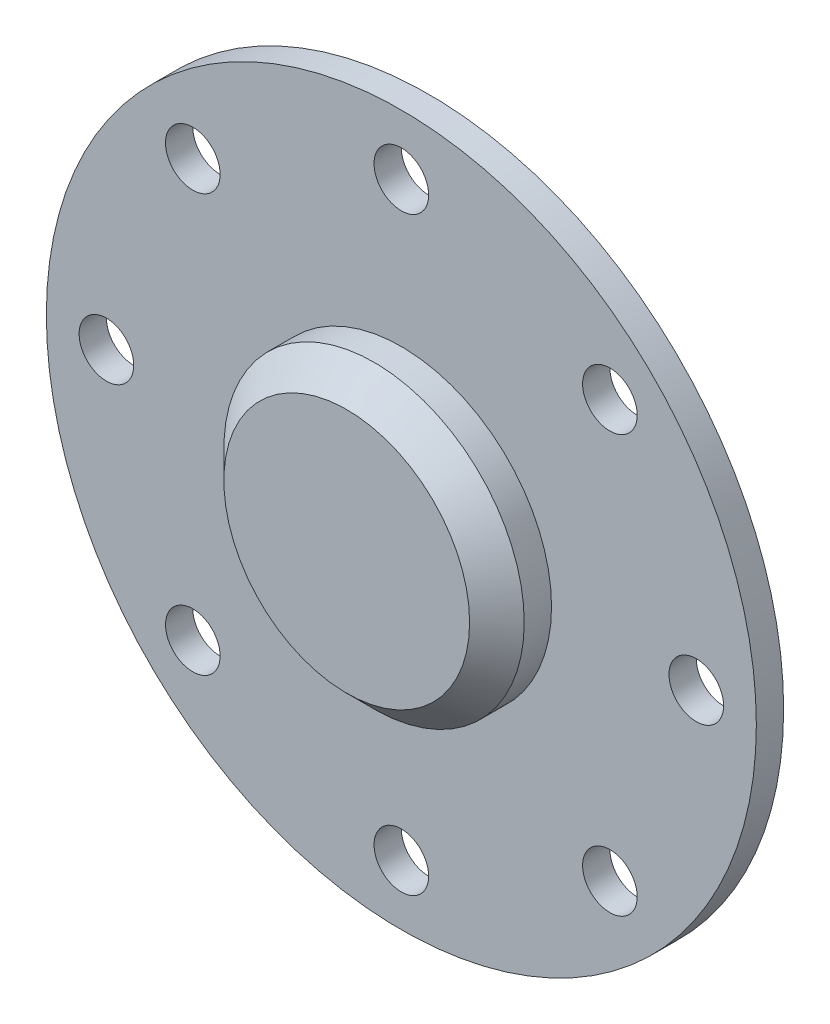
from build123d import *

# Parameters (mm, degrees)
SKETCH_1_R          = 130
SKETCH_1_R_2        = 10
EXTRUDE_1_DEPTH     = 10
SKETCH_2_R          = 55
EXTRUDE_2_DEPTH     = 20
SKETCH_3_R          = 45
CUT_EXTRUDE_1_DEPTH = 20
CHAMFER_1_SIZE      = 10


with BuildPart() as part:
    # 草图1 → 凸台-拉伸1 (new body)
    with BuildSketch(Plane.XY):
        Circle(SKETCH_1_R)
        with Locations((0, 108)):
            Circle(SKETCH_1_R_2, mode=Mode.SUBTRACT)
        with Locations((76.367532368, 76.367532368)):
            Circle(SKETCH_1_R_2, mode=Mode.SUBTRACT)
        with Locations((108, 0)):
            Circle(SKETCH_1_R_2, mode=Mode.SUBTRACT)
        with Locations((76.367532368, -76.367532368)):
            Circle(SKETCH_1_R_2, mode=Mode.SUBTRACT)
        with Locations((0, -108)):
            Circle(SKETCH_1_R_2, mode=Mode.SUBTRACT)
        with Locations((-76.367532368, -76.367532368)):
            Circle(SKETCH_1_R_2, mode=Mode.SUBTRACT)
        with Locations((-108, 0)):
            Circle(SKETCH_1_R_2, mode=Mode.SUBTRACT)
        with Locations((-76.367532368, 76.367532368)):
            Circle(SKETCH_1_R_2, mode=Mode.SUBTRACT)
    extrude(amount=EXTRUDE_1_DEPTH)

    # 草图2 → 凸台-拉伸2 (add)
    with BuildSketch(Plane.XY.offset(10)):
        Circle(SKETCH_2_R)
    extrude(amount=EXTRUDE_2_DEPTH)

    # 草图3 → 切除-拉伸1 (cut)
    with BuildSketch(Plane(origin=(0, 0, 0), x_dir=(-1, 0, 0), z_dir=(0, 0, -1))):
        Circle(SKETCH_3_R)
    extrude(amount=-CUT_EXTRUDE_1_DEPTH, mode=Mode.SUBTRACT)

    # 倒角1
    chamfer_1_edges = [part.edges().sort_by_distance(p)[0] for p in [
        (-55, 0, 30),
    ]]
    chamfer(chamfer_1_edges, length=CHAMFER_1_SIZE)


solid = part.part
